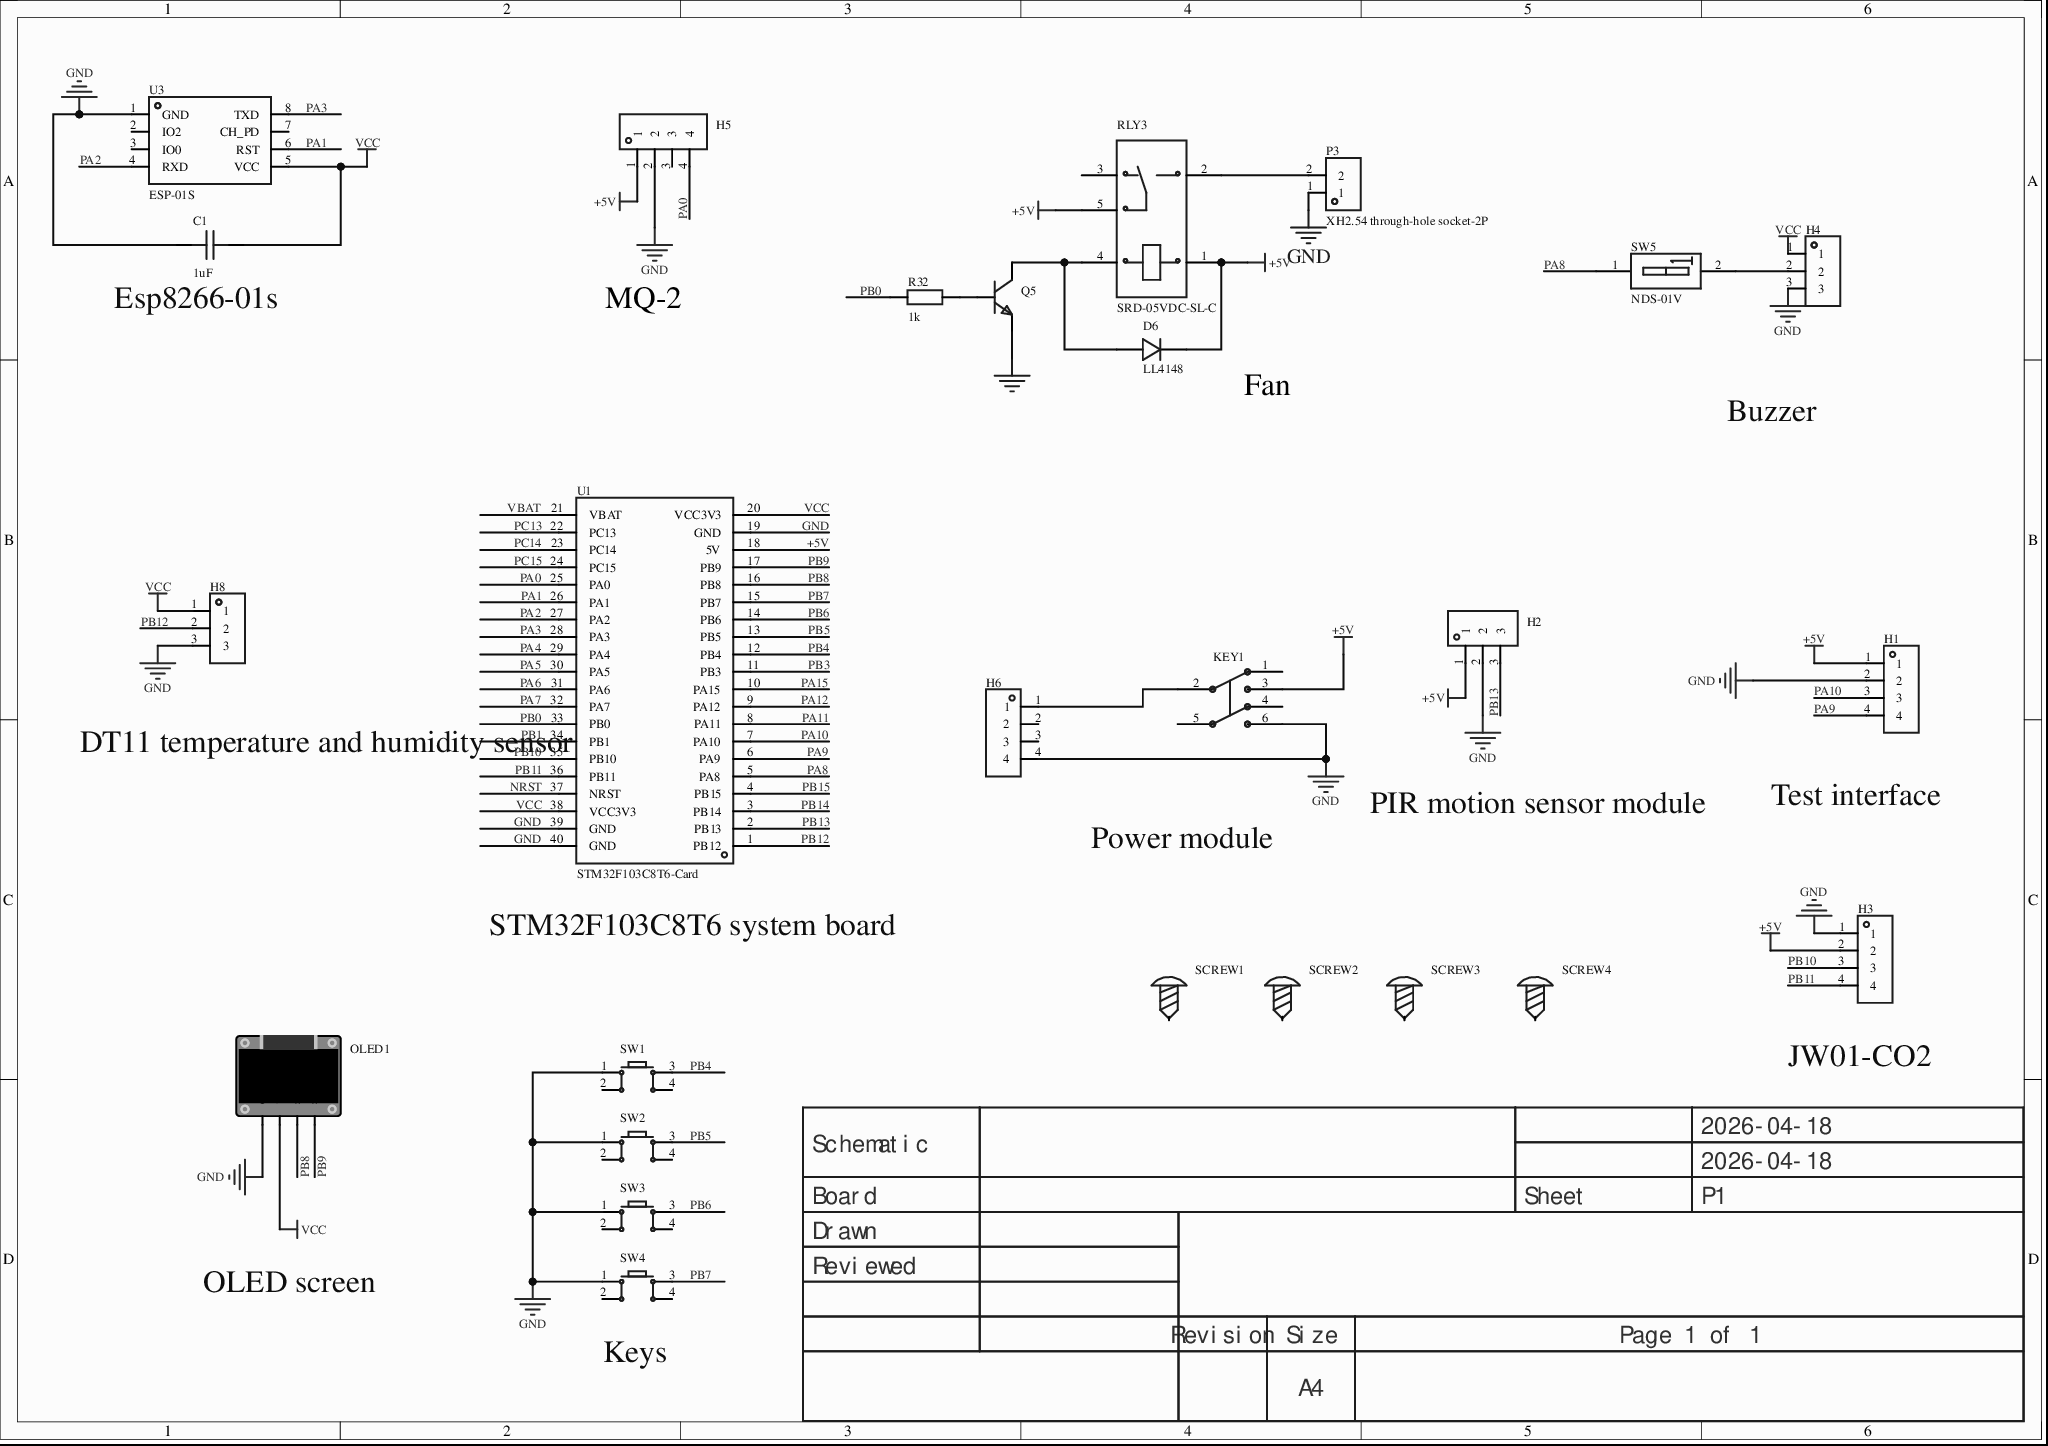
[diagram p0: MISC75114-3.schdoc]
# Altium project MISC75114-2.PrjPcb
1 sheet, 26 parts. Net scope: global (net labels, ports and power ports of the same name join across sheets).
Board file: MISC75114.pcbdoc

## Sheet MISC75114-3.schdoc
size 297 x 209 mm; Version: V1.0; @Project Name: MISC75114; @Page Count: 1; @Update Date: 2026-04-18; @Create Date: 2026-04-18; @Schematic Name: MISC75114; @Page No: 1; @Create Time: 18:58:15; @Update Time: 22:44:58; @Board Name: MISC75114

### Parts
C1  1uF  [C0603]
D6  LL4148  [LL-34_L3.5-W1.5-RD]
H1  (no value)  [HDR-TH_4P-P2.54-V-M]
H2  (no value)  [HDR-TH_3P-P2.54-V-F]
H3  (no value)  [HDR-TH_4P-P2.54-V-M]
H4  (no value)  [HDR-TH_3P-P2.54-V-F]
H5  (no value)  [HDR-TH_4P-P2.54-V-F]
H6  (no value)  [HDR-TH_4P-P2.54-V-F]
H8  (no value)  [HDR-TH_3P-P2.54-V-F]
KEY1  Non-latching switch 8.5×8.5 silent  [SW-TH_6P-L8.5-W8.5-P2.54]  (value not drawn)
OLED1  (no value)  [0.96OLED_4P]
P3  XH2.54 through-hole socket-2P  [CONN-TH_XH2.54-2P]
Q5  (no value)  [S8050_SOT-23]
R32  1k  [R0603]
RLY3  SRD-05VDC-SL-C  [RELAY-TH_SRD-XXVDC-XL-C]
SCREW1  (no value)  [M3螺丝]
SCREW2  (no value)  [M3螺丝]
SCREW3  (no value)  [M3螺丝]
SCREW4  (no value)  [M3螺丝]
SW1  (no value)  [SW-TH_4P-L6.0-W6.0-P4.50-LS6.5]
SW2  (no value)  [SW-TH_4P-L6.0-W6.0-P4.50-LS6.5]
SW3  (no value)  [SW-TH_4P-L6.0-W6.0-P4.50-LS6.5]
SW4  (no value)  [SW-TH_4P-L6.0-W6.0-P4.50-LS6.5]
SW5  NDS-01V  [SW-TH_2P-L3.9-W9.9-P2.54-LS7.6]
U1  STM32F103C8T6-Card  [CONN-TH_L53.3-W22.9_STM32F103C8T6-CARD]
U3  ESP-01S  [WIFIM-TH_ESP-01S]

### Nets
+5V: D6.1(K) H1.1 H2.1 H3.2 H5.1 KEY1.3 RLY3.1 RLY3.5 U1.18(5V)
GND: C1.1 H1.2 H2.2 H3.1 H4.3 H5.2 H6.4 H8.3 KEY1.6 OLED1.1(GND) P3.1 Q5.2 SW1.1 SW2.1 SW3.1 SW4.1 U1.19(GND) U1.39(GND) U1.40(GND) U3.1(GND)
VCC: C1.2 H4.1 H8.1 OLED1.2(VCC) U1.20(VCC3V3) U1.38(VCC3V3) U3.5(VCC)
NRST: U1.37(NRST)
PA0: H5.4 U1.25(PA0)
PA1: U1.26(PA1) U3.6(RST)
PA2: U1.27(PA2) U3.4(RXD)
PA3: U1.28(PA3) U3.8(TXD)
PA4: U1.29(PA4)
PA5: U1.30(PA5)
PA6: U1.31(PA6)
PA7: U1.32(PA7)
PA8: SW5.1(A1) U1.5(PA8)
PA9: H1.4 U1.6(PA9)
PA10: H1.3 U1.7(PA10)
PA11: U1.8(PA11)
PA12: U1.9(PA12)
PA15: U1.10(PA15)
PB0: R32.1 U1.33(PB0)
PB1: U1.34(PB1)
PB3: U1.11(PB3)
PB4: SW1.3 U1.12(PB4)
PB5: SW2.3 U1.13(PB5)
PB6: SW3.3 U1.14(PB6)
PB7: SW4.3 U1.15(PB7)
PB8: OLED1.3(SCL) U1.16(PB8)
PB9: OLED1.4(SDA) U1.17(PB9)
PB10: H3.3 U1.35(PB10)
PB11: H3.4 U1.36(PB11)
PB12: H8.2 U1.1(PB12)
PB13: H2.3 U1.2(PB13)
PB14: U1.3(PB14)
PB15: U1.4(PB15)
PC13: U1.22(PC13)
PC14: U1.23(PC14)
PC15: U1.24(PC15)
VBAT: U1.21(VBAT)
NetD6_2: D6.2(A) Q5.3 RLY3.4
NetH4_2: H4.2 SW5.2(A2)
NetH6_1: H6.1 KEY1.2
NetP3_2: P3.2 RLY3.2
NetQ5_1: Q5.1 R32.2

Not connected (* = marked no-connect by the designer): H5 3*; H6 2 3; KEY1 1 4 5; RLY3 3*; SCREW1 1; SCREW2 1; SCREW3 1; SCREW4 1; SW1 2 4; SW2 2 4; SW3 2 4; SW4 2 4; U3 2(IO2)* 3(IO0)* 7(CH_PD)*

### Notes on the sheet
- (near C1) Esp8266-01s
- MQ-2
- Fan
- Buzzer
- (near U1) DT11 temperature and humidity sensor
- Power module
- PIR motion sensor module
- (near H1) Test interface
- (near U1) STM32F103C8T6 system board
- (near H3) JW01-CO2
- OLED screen
- (near SW4) Keys
- 2026-04-18
- Schematic
- Board
- Sheet
- P1
- Drawn
- Reviewed
- Revision
- Size
- A4
- Page 1 of 1

### Library data of the parts
C1 = CAP_0603: Symbol: Capacitance; ConvertToPcb: yes; ModelId: ac125912035d415993ca9572d50418b10819f05c4eef4c71ace90d822a990e87; ModelName: C0603_L1.6-W0.8-H0.8; ModelTransform: 62.992,31.496,0,0,0,0,0,0,0; Device: CAP_0603; Value: 1uF; AddInBom: yes; Supplier Footprint: 0603; FootprintName: C0603
D6 = LL4148_C9808: 二极管配置:-;功率:500mW;直流反向耐压(Vr):75V;平均整流电流(Io):200mA;正向压降(Vf):1V@10mA;反向电流(Ir):5uA@75V;反向恢复时间(trr):4ns;工作温度:+175℃@(Tj);; Manufacturer: ST(先科); 3D Model: 4a6f2309ca4c4217857da1816cccdf69; 3D Model Transform: 133.93674,59.031,0,0,0,0,0,0,0; Power Dissipation: 500mW; Reverse Voltage (Vr): 75V; Average Rectified Current (Io): 200mA; Reverse Recovery Time (trr): 4ns; AddInBom: yes; ModelName: LL-34_L3.5-W1.5; Symbol: LL4148; Device: LL4148_C9808; LCSC Part Name: 75V 200mA 4ns; Supplier Part: C9808; Manufacturer Part: LL4148; Supplier Footprint: LL-34; JLCPCB Part Class: Basic library; Datasheet: https://atta.szlcsc.com/upload/public/pdf/source/20121108/1457706554347.pdf; Supplier: LCSC; Diode Configuration: -; Forward Voltage (Vf@If): 1V@10mA; Reverse Leakage Current: 5uA@75V; Operating Temperature: +175℃@(Tj); ConvertToPcb: yes; FootprintName: LL-34_L3.5-W1.5-RD
H1 = HDR-M_2.54_1x4P: Symbol: PZ254V-11-04P; ConvertToPcb: yes; ModelId: 112f4d05e8d64e99ab9a333894bea4f90819f05c4eef4c71ace90d822a990e87; ModelName: HDR-TH_4P-P2.54-M-LI-1X4P; ModelTransform: 399.999,104.7242,0,0,0,0,0,0,-118.11; Device: HDR-M_2.54_1x4P; AddInBom: yes; SupplierPart: C492403; Supplier Footprint: 插件; FootprintName: HDR-TH_4P-P2.54-V-M
H2 H4 H8 = HDR-F_2.54_1x3P: Symbol: PM254V-11-03-H85; 3D Model: f3b3cc5aae9641bf9e56fc160cef875b; 3D Model Transform: 299.9994,100,0,0,0,0,0,0,-118.11; ConvertToPcb: yes; ModelName: HDR2.54-F-LI-1X3P; Device: HDR-F_2.54_1x3P; Supplier Part: C541850; Supplier Footprint: 插件; AddInBom: yes; FootprintName: HDR-TH_3P-P2.54-V-F
H3 = HDR-M_2.54_1x4P: Symbol: PZ254V-11-04P; 3D Model: 112f4d05e8d64e99ab9a333894bea4f90819f05c4eef4c71ace90d822a990e87; 3D Model Transform: 399.999,104.7242,0,0,0,0,0,0,-118.11; ConvertToPcb: yes; ModelName: HDR-TH_4P-P2.54-M-LI-1X4P; Device: HDR-M_2.54_1x4P; Supplier Part: C492403; Supplier Footprint: 插件; AddInBom: yes; FootprintName: HDR-TH_4P-P2.54-V-M
H5 = HDR-F_2.54_1x4P: Symbol: 2.54-1*4P female; ConvertToPcb: yes; ModelId: d187812051054f85879fcaa51a310d8e0819f05c4eef4c71ace90d822a990e87; ModelTransform: 419.6842,98.464,0,0,0,0,0,0,-118.11; Device: HDR-F_2.54_1x4P; AddInBom: yes; SupplierPart: C2718488; Supplier Footprint: 插件; FootprintName: HDR-TH_4P-P2.54-V-F; ModelName: HDR-TH_4P-P2.54-V-F
H6 = HDR-F_2.54_1x4P: Symbol: 2.54-1*4P female; 3D Model: d187812051054f85879fcaa51a310d8e0819f05c4eef4c71ace90d822a990e87; 3D Model Transform: 419.6842,98.464,0,0,0,0,0,0,-118.11; ConvertToPcb: yes; Device: HDR-F_2.54_1x4P; Supplier Part: C2718488; Supplier Footprint: 插件; AddInBom: yes; FootprintName: HDR-TH_4P-P2.54-V-F; ModelName: HDR-TH_4P-P2.54-V-F
KEY1 = 无自锁开关 8.5×8.5 无声: 6 pins, 8.5×8.5; Symbol: No self-locking switch 8.5×8.5 silent; AddInBom: yes; ModelId: 4c72b3966b92446eb355e1bd0fb4f8800819f05c4eef4c71ace90d822a990e87; ModelTransform: 342.519,334.645,0,180,0,0,0,0,-137.795; Device: Non-latching switch 8.5×8.5 silent; LCSC Part Name: 无自锁开关 8.5×8.5  无声; SupplierPart: C26228; ManufacturerPart: 无自锁开关 8.5×8.5 无声; Supplier Footprint: 插件; JLCPCB Part Class: Extended Part; Supplier: LCSC; ConvertToPcb: yes; FootprintName: SW-TH_6P-L8.5-W8.5-P2.54; ModelName: SW-TH_6P-L8.5-W8.5-P2.54
OLED1 = 0.96OLED模块_4P: Symbol: 0.96OLED module_4P; ConvertToPcb: yes; ModelId: 79c000fdb68d45a296c2e9bedf4f9055; ModelTransform: 1393.69792,1318.895,0,0,0,0,0,-560.079,-137.795; Device: 0.96OLED module_4P; AddInBom: yes; FootprintName: 0.96OLED_4P; Supplier Footprint: 插件; ModelName: 0.96OLED_4P
P3 = XH2.54直插座-2P: 3D Model: dc9654a6caad4c20aab3bc231ea458cf; 3D Model Transform: 296.889,230.315,0,0,0,0,0,26.653,-137.795; AddInBom: yes; Symbol: XH2.54 through-hole socket-2P; Device: XH2.54 through-hole socket-2P; LCSC Part Name: XH2.54直插座-2P; Supplier Part: C9900016957; Manufacturer Part: XH2.54直插座-2P; Supplier Footprint: XH2.54-2; JLCPCB Part Class: Extended library; Supplier: LCSC; ConvertToPcb: yes; FootprintName: CONN-TH_XH2.54-2P; ModelName: CONN-TH_XH2.54-2P
Q5 = S8050_SOT_NPN: Symbol: NPN; 3D Model: c62791f0466c4ae2a892c056b845b0ca; 3D Model Transform: 98.6,114.12,41.29,180,0,0,0,0,-3; ConvertToPcb: yes; ModelName: SOT-23-3P_L2.9-W1.3-H1.0-LS2.4-P0.95; Device: S8050_SOT_NPN; Supplier Footprint: SOT-23; AddInBom: yes; FootprintName: S8050_SOT-23
R32 = Res_0603: Symbol: Resistor; 3D Model: fc143cca1e79419f9cd78b61e9279f08; 3D Model Transform: 31.8897,63.7794,0,90,0,0,0,0,0; ConvertToPcb: yes; Device: Res_0603; Value: 1k; Supplier Footprint: 0603; AddInBom: yes; FootprintName: R0603; ModelName: R0603
RLY3 = SRD-05VDC-SL-C: Coil voltage:5V;Contact form:1C (SPDT) changeover;Contact capacity (resistive load):-;Max switching voltage:250V@AC;Max switching current:15A;; Manufacturer: 松乐; 3D Model: d0eda9b8bf8746d18ae810ab88dc78e7; 3D Model Transform: 755.904,622.4397,0,0,0,0,34.882,0,-118.11; Coil Voltage: 5V; Pin Number: 5; Coil Rated Power: 360mW; Maximum Switching Current: 15A; Coil Type: Non-polar, single coil; Coil Resistance: 70Ω; Contact Resistance: 100mΩ; Operate Time: 10ms; AddInBom: yes; ModelName: RELAY-TH_L19.2-W15.6-H15.8; Symbol: SRD-05VDC-SL-C; Device: SRD-05VDC-SL-C; LCSC Part Name: 蓝色; Supplier Part: C35449; Manufacturer Part: SRD-05VDC-SL-C; Supplier Footprint: 插件,15.6x19.2mm; JLCPCB Part Class: Extended library; Datasheet: https://atta.szlcsc.com/upload/public/pdf/source/20200305/C490149_C96E4098A3B1FFB377D5AD2E40B7C2A8.pdf; Supplier: LCSC; Contact Form: 1C (SPDT) changeover; Contact Rating: -; Maximum Switching Voltage: 250V@AC; Release Time: 10ms; ConvertToPcb: yes; FootprintName: RELAY-TH_SRD-XXVDC-XL-C
SCREW1-SCREW4 = M3螺丝: Symbol: Screw hole; Device: M3 screw; ConvertToPcb: yes; AddInBom: yes; Supplier Footprint: 插件; FootprintName: M3 screw
SW1-SW4 = Key_TH_6x6x6: 触点电流:50mA;额定电压(DC):12V;绝缘电阻:100MΩ;电路结构:单刀单掷;安装方式:直插;按钮形状:圆形按钮;按钮/盖帽颜色:黑色;作用力:260gf@±30gf;工作温度:-25℃~+70℃;引脚样式:PC引脚;开关长度:6mm;开关宽度:6mm;开关高度:6mm;带支架:否;; Symbol: Tact switch; AddInBom: yes; ModelId: 20eee248bc684ccd8cbdbb1d0d91ec6f0819f05c4eef4c71ace90d822a990e87; ModelName: SW-TH_4P-L6.0-W6.0-H5.0-LS6.5-P4.50; ModelTransform: 236.22,323.03,0,90,0,0,0,0,-137.795; Device: Key_TH_6x6x6; ConvertToPcb: yes; FootprintName: SW-TH_4P-L6.0-W6.0-P4.50-LS6.5; Supplier Footprint: 插件
SW5 = NDS-01V_C501305: Forward-action high lever; 3D Model: a6fe51954c31461ebc9e88beb6e51f3d0819f05c4eef4c71ace90d822a990e87; 3D Model Transform: 161.417,389.763,0,270,0,0,0,0,-125.984; AddInBom: yes; ModelName: SW-TH_L4.0-W9.9-H5.4-P2.54-B; Symbol: NDS-01V; Device: NDS-01V_C501305; LCSC Part Name: 拨码开关; Supplier Part: C501305; Manufacturer Part: NDS-01V; Supplier Footprint: DIP; JLCPCB Part Class: Extended Part; Supplier: LCSC; ConvertToPcb: yes; FootprintName: SW-TH_2P-L3.9-W9.9-P2.54-LS7.6
U1 = STM32F103C8T6-Card: AddInBom: yes; Symbol: STM32F103C8T6-CARD; Device: STM32F103C8T6-Card; LCSC Part Name: STM32F103C8T6-Card; SupplierPart: C9900077949; ManufacturerPart: STM32F103C8T6-Card; Supplier Footprint: 插件; Supplier: LCSC; ConvertToPcb: yes; FootprintName: CONN-TH_L53.3-W22.9_STM32F103C8T6-CARD
U3 = ESP-01S_C111009: 3D Model: eb7175da78ae48b3b1568cfe3027405f0819f05c4eef4c71ace90d822a990e87; 3D Model Transform: 582.676,976.37608,0,0,0,0,0,388.346,-118.11; AddInBom: yes; Symbol: ESP-01S; Device: ESP-01S_C111009; LCSC Part Name: ESP-01S; Supplier Part: C111009; Manufacturer Part: ESP-01S; Supplier Footprint: -; JLCPCB Part Class: Extended Part; Supplier: LCSC; ConvertToPcb: yes; FootprintName: WIFIM-TH_ESP-01S; ModelName: WIFIM-TH_ESP-01S